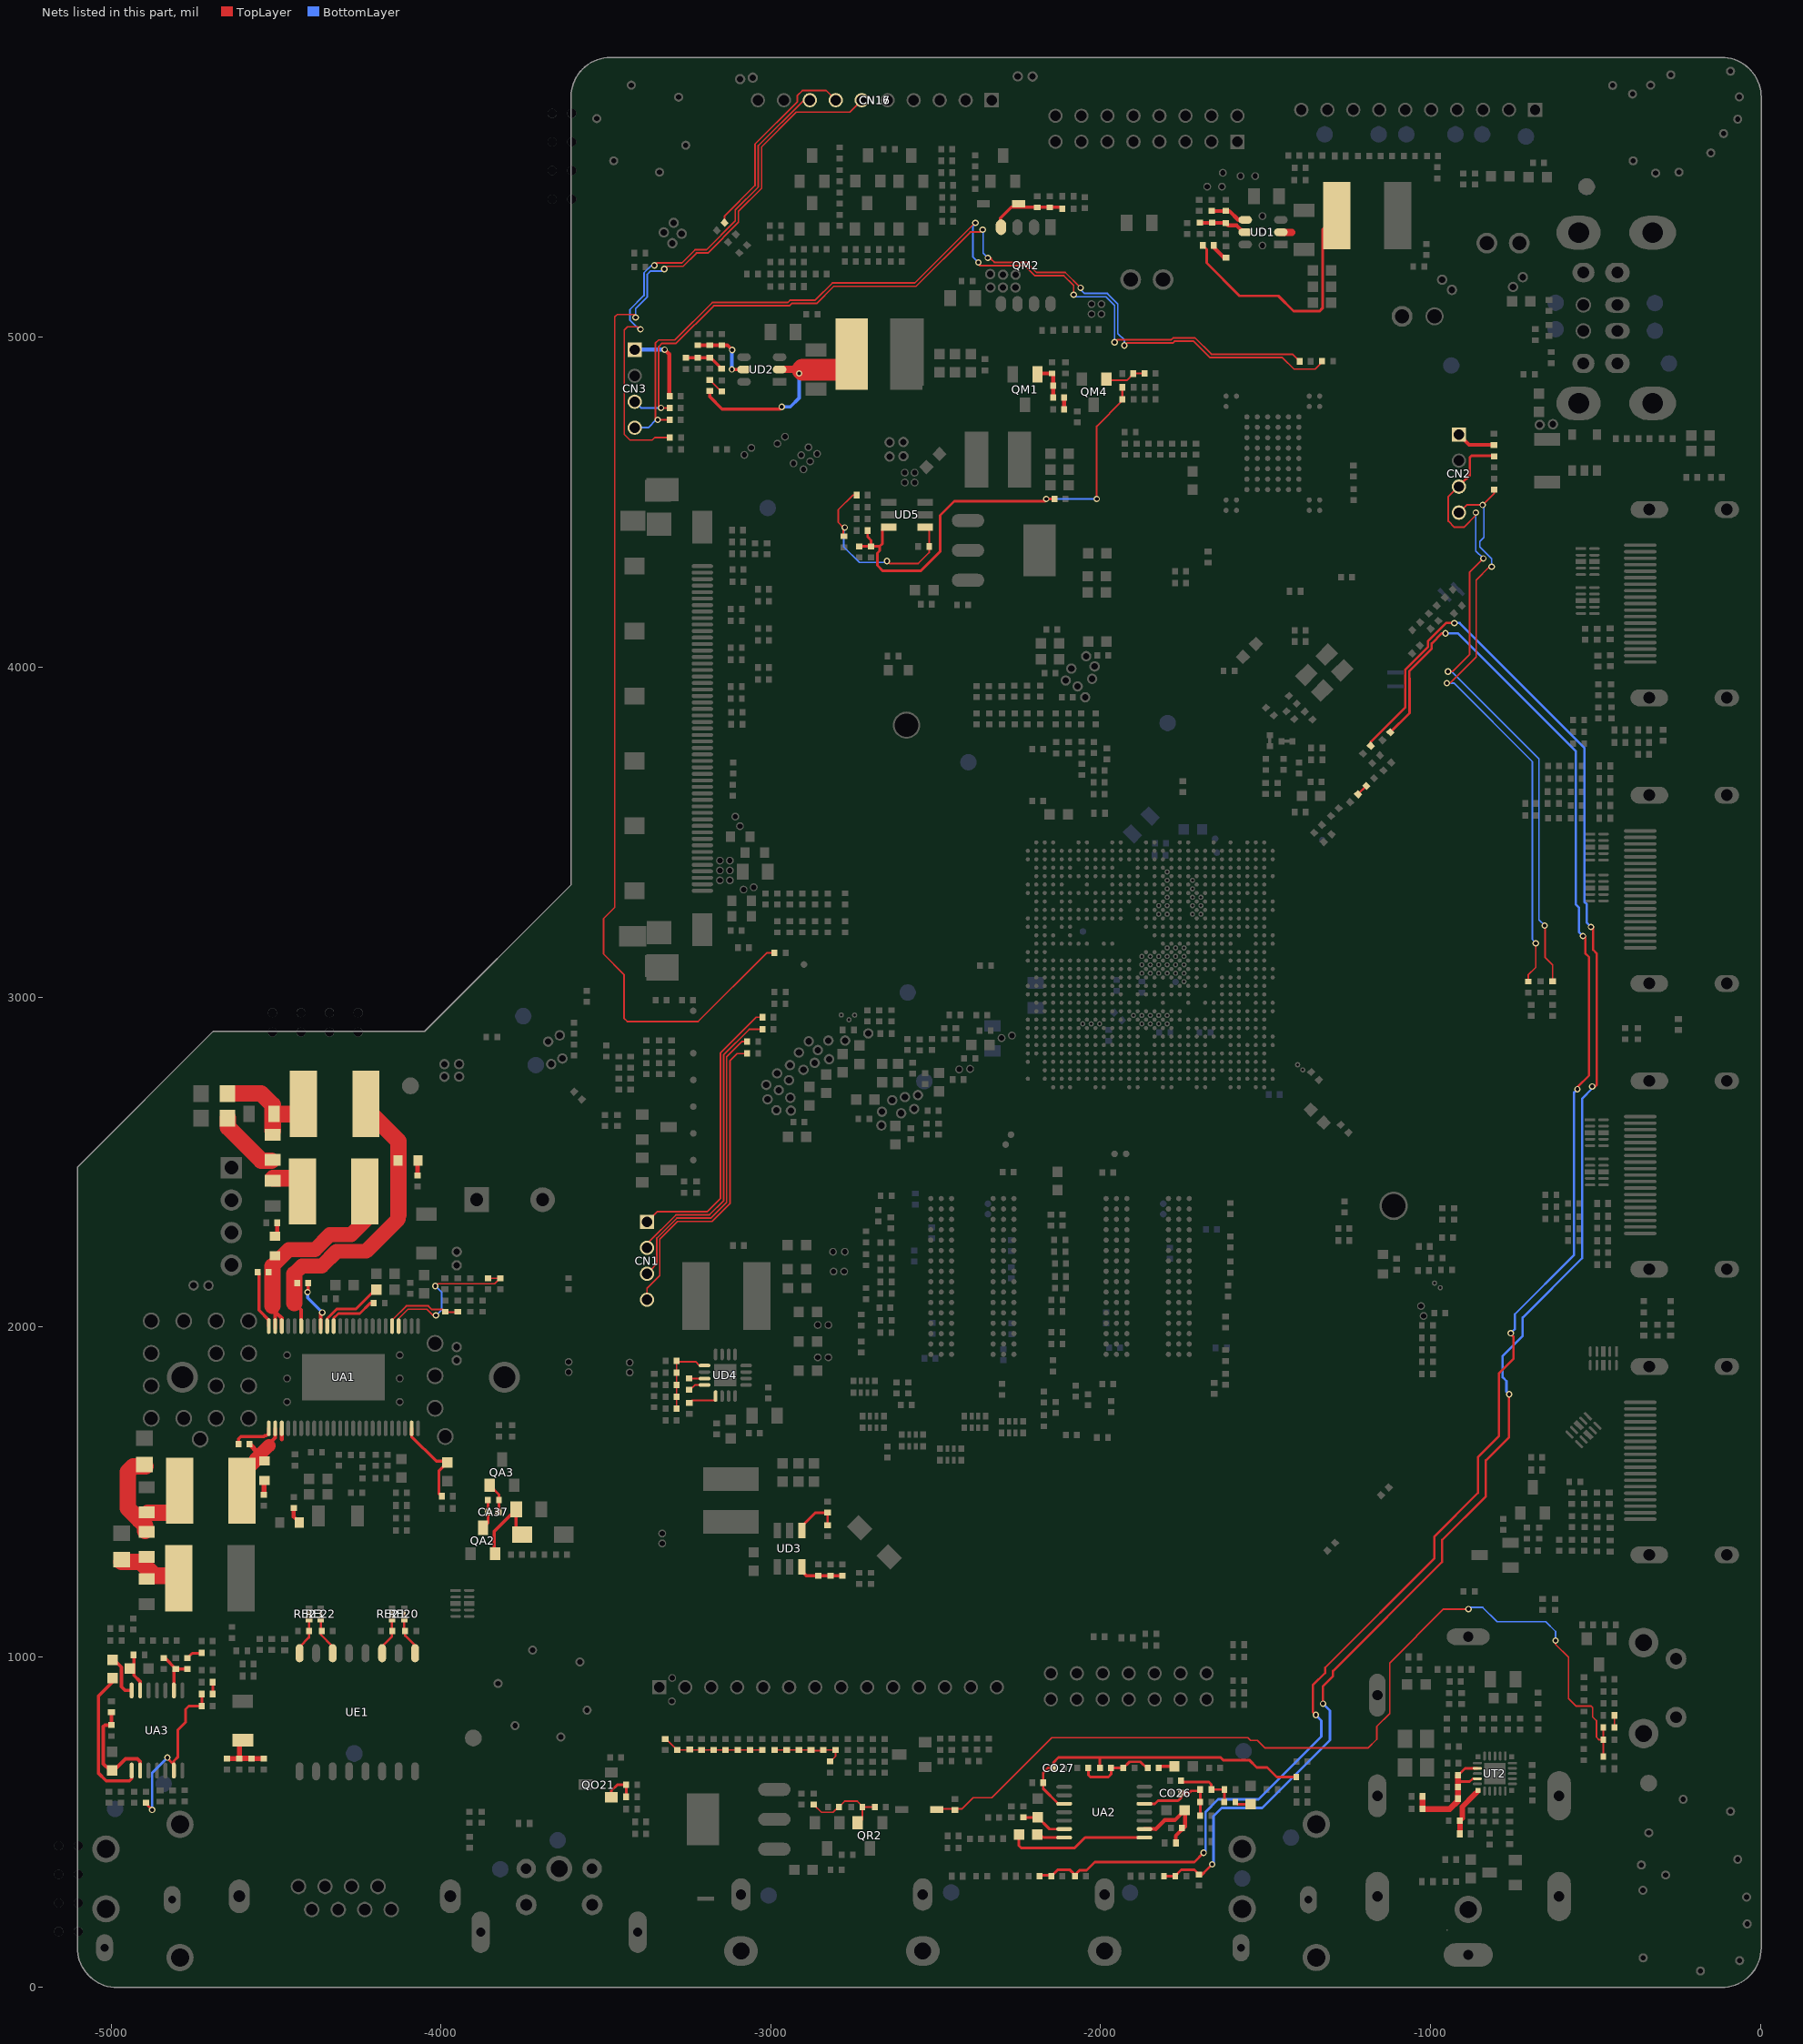
[diagram p0: the nets of this part, all layers, seen from the top]
# Altium PCB MISC86290.PcbDoc (part 25 of 31)
Units mil, origin at the board's own origin, x right, y up, seen from the top; angles counter-clockwise.
Board outline 5104.71 x 5851.49 mil, 2 copper layers (TopLayer, BottomLayer), stack 61.855 mil thick; 1026 components, 667 nets, 4280 pads, 2294 vias.

## Via types
v1: diameter 19.68, hole 11.81, TopLayer to BottomLayer, tented both sides, 1189 vias
v2: diameter 19.68/19.68 (per signal layer), hole 11.81, TopLayer to BottomLayer, tented both sides, 366 vias
v3: diameter 15.75, hole 7.87, TopLayer to BottomLayer, tented both sides, 348 vias
v4: diameter 23.62, hole 15.75, TopLayer to BottomLayer, tented both sides, 309 vias
v5: diameter 15.75/15.75 (per signal layer), hole 7.87, TopLayer to BottomLayer, tented both sides, 59 vias
v6: diameter 24/24 (per signal layer), hole 16, TopLayer to BottomLayer, tented both sides, 23 vias

## Nets (pads, with @x,y where several pads share a name; then routed paths per layer and width w, separated by ;. In a path a pad name is that pad's centre, name@x,y a point inside that pad or via, vN(x,y) a via of type N, cw(c..) or ccw(c..) an arc to the next point about the centre after c; other vN are vias at no path point) (continued)
NetCA14_1: CA14.1 CA18.2 LA1.2 RA30.1 | length 190.3
  TopLayer w50: RA30.1@-4968,1288.23 -4910.23,1288.23 -4868,1246 LA1.2@-4795.23,1246
NetCA17_1: CA17.1 CA18.1 LA2.2 RA31.1 | length 503.8
  TopLayer w50: CA18.1@-4897,1382.03 -4897,1398 -4912,1413 ; RA31.1@-4896,1577 -4899.01,1577 -4933,1577 -4949.17,1560.83 -4949.17,1450.17 -4914.5,1415.5 -4912,1413 ; LA2.2@-4791.88,1565.21 LA2.2@-4791.88,1503.52 -4791.88,1462.12 -4817,1437 -4888,1437 -4889.53,1435.47 -4912,1413
NetCA19_1: CA19.1 UA1.1 | length 129.8
  TopLayer w10: CA19.1@-4613.73,1645 -4613.73,1661.27 -4607,1668 -4536.43,1668 -4534.27,1670.17 -4529.51,1670.17 -4522.13,1677.55 UA1.1@-4522.13,1692.73
NetCA19_2: CA19.2 LA2.1 RA17.1 UA1.2 UA1.3 | length 203.6
  TopLayer w11.8: -4517.18,1649.37 -4502.44,1664.1 UA1.2@-4502.44,1692.73 ; -4482.76,1659.31 UA1.3@-4482.76,1692.73
  TopLayer w15: CA19.2@-4580.27,1645 -4554.69,1619.42
  TopLayer w40: LA2.1@-4577.55,1578.68 -4562.91,1593.33 -4562.91,1599.1 -4521.84,1640.17
NetCA20_1: CA20.1 CA21.2 UA1.23 | length 291.3
  TopLayer w9: UA1.23@-4089.06,1681.87 -4089.06,1668.06 -4014,1593 -3987.62,1593 CA21.2@-3981,1599.62 ; CA20.1@-3997.73,1487 -4006.5,1495.77 -4006.5,1563.12 CA21.2@-3981,1588.62
  TopLayer w10: UA1.23@-4089.06,1672.96 -4089.06,1681.87 UA1.23@-4089.06,1692.73
NetCA22_1: CA22.1 UA1.48 | length 171.5
  TopLayer w10: CA22.1@-4551.73,2162 -4551.73,2050.73 -4522.13,2021.13 UA1.48@-4522.13,2002.77
NetCA22_2: CA22.2 LA3.2 RA18.1 UA1.46 UA1.47 | length 714.5
  TopLayer w11.8: -4511,2064 -4511,2055.19 -4498.2,2042.39 ; UA1.47@-4502.44,1994.89 UA1.47@-4502.44,2023.63 ; UA1.47@-4502.44,2002.77 -4502.44,2038.15 -4498.2,2042.39 ; UA1.46@-4482.76,1994.89 UA1.46@-4482.76,2002.77 -4482.76,2026.94 -4498.2,2042.39
  TopLayer w45: -4511,2184.5 -4461,2234.5 -4382.23,2234.5 -4336.98,2279.75 -4272.25,2279.75 -4228.51,2323.49 LA3.2@-4228.51,2426.5
  TopLayer w50: -4511,2064 -4511,2184.5
NetCA23_1: CA23.1 UA1.38 | length 168.3
  TopLayer w8: UA1.38@-4325.28,2002.77 -4325.28,2026.84 -4311.12,2041 -4246,2041 -4215,2072 CA23.1@-4203.73,2072
  TopLayer w10: UA1.38@-4325.28,1994.89 UA1.38@-4325.28,1998.83
NetCA24_1: CA24.1 CA26.1 LA3.1 RA32.1 | length 291.5
  TopLayer w50: RA32.1@-4646,2633 -4646,2632.59 -4646,2605.5 -4544.5,2504 CA24.1@-4513.33,2504 ; CA26.1@-4508.77,2451.04 LA3.1@-4419.5,2451.04
NetCA24_2: CA24.2 CA27.1 LA4.2 RA33.1 | length 347.2
  TopLayer w50: -4618.5,2708 -4545,2708 -4510.36,2673.36 -4510.36,2646.5 CA24.2@-4510.36,2595 ; CA27.1@-4506.97,2645.5 -4505.97,2645.5 -4435,2645.5 -4413.49,2667.01 -4413.49,2676.38 LA4.2@-4413.49,2711
NetCA25_1: CA25.1 UA1.39 | length 209.9
  TopLayer w8: UA1.39@-4344.96,2002.77 -4344.96,2025.54 -4316.5,2054 -4258.57,2054 -4195.81,2116.76 CA25.1@-4195.81,2117
NetCA28_1: CA28.1 UA1.40 | length 160.4
  TopLayer w10: v1(-4404.27,2105.73) -4402.27,2105.73 CA28.1@-4402.27,2133 ; UA1.40@-4364.65,1994.89 UA1.40@-4364.65,2002.77 -4364.65,2039.35 v1(-4360,2044)
  BottomLayer w10: v1(-4404.27,2105.73) -4404.27,2088.27 v1(-4360,2044)
NetCA28_2: CA28.2 LA4.1 RA19.1 UA1.43 | length 917.2
  TopLayer w11: -4445,2072.84 -4423.7,2051.55 UA1.43@-4423.7,2002.77
  TopLayer w45: -4445,2161 -4421.5,2184.5 -4361.51,2184.5 -4316.27,2229.75 -4227.02,2229.75 -4129,2327.77 -4129,2339.95
  TopLayer w50: -4445,2072.84 -4445,2161 ; LA4.1@-4224.51,2645.95 -4211.95,2645.95 -4129,2563 -4129,2339.95
NetCA32_1: CA32.1 RA16.2 | length 50.2
  TopLayer w12: CA32.1@-4446.39,1450.79 -4446.39,1424.3 RA16.2@-4429.61,1407.52
NetCA33_1: CA33.1 RA17.2 | length 37.5
  TopLayer w15: CA33.1@-4536.39,1499.52 RA17.2@-4536.39,1537.01
NetCA34_1: CA34.1 RA18.2 | length 33.5
  TopLayer w12: RA18.2@-4496.04,2282.52 CA34.1@-4496.04,2316.01
NetCA35_1: CA35.1 RA19.2 | length 44.5
  TopLayer w15: CA35.1@-4071,2459.73 RA19.2@-4071,2504.22
NetCA36_2: CA36.2 DA9.K QA2.E | length 248.8
  TopLayer w10: QA2.E@-3838.5,1308 -3838.5,1380.53 CA36.2@-3772.03,1447 -3772.03,1386.04 DA9.K@-3756.99,1371
NetCA37_1: CA37.1 QA2.C RA23.1 | length 90.1
  TopLayer w8: QA2.C@-3872.5,1391.03 -3857.73,1405.8 CA37.1@-3857.73,1439 RA23.1@-3857.73,1475
NetCA37_2: CA37.2@-3824.26,1439 CA37.2@-3831.15,1439 QA3.B RA23.2 | length 92.7
  TopLayer w8: QA3.B@-3852.5,1520 -3824.27,1491.77 RA23.2@-3824.27,1475 CA37.2@-3824.26,1439
NetCA38_2: CA38.2 RA14.2 UA1.29 | length 243
  TopLayer w5: UA1.29@-4148.11,2002.77 -4148.11,2021.89 -4145,2025 -4144.18,2025 -4105.18,2064 -4038.14,2064 -4027.14,2053 -3993.73,2053 CA38.2@-3987,2046.27 ; CA38.2@-3987,2045.27 RA14.2@-3949,2045.27
NetCA39_2: CA39.2 RA12.2 UA1.28 | length 508.6
  TopLayer w5: UA1.28@-4128.43,2002.77 -4128.43,2025.57 -4100,2054 -4043,2054 -4024,2035 v1(-4015,2035) v1@-4015,2040 ; v1(-4017,2124) -4010,2131 -3837.11,2131 CA39.2@-3820.35,2147.76 RA12.2@-3857.35,2147.76
  BottomLayer w5: v1(-4017,2124) -3997.66,2104.66 -3997.66,2052.34 v1(-4015,2035)
NetCA53_2: CA53.2 RO31.2 RO33.1 UA3.2 | length 153.7
  TopLayer w10: RO33.1@-4840.84,996.73 -4837.3,996.73 CA53.2@-4803.84,963.27 ; UA3.2@-4809.73,898.32 -4809.73,957.37 CA53.2@-4803.84,963.27 ; RO31.2@-4768.34,963.27 CA53.2@-4803.84,963.27
NetCA56_2: CA56.2 RO32.2 RO34.1 UA3.13 | length 531.3
  TopLayer w8: RO34.1@-4892.77,559 RO34.1@-4894.5,557.27 -4894.5,555 v1(-4875.5,536) ; v1(-4829.5,694.5) -4829.5,692.68 UA3.13@-4809.73,672.92 ; UA3.13@-4809.73,655.21 UA3.13@-4809.73,672.92 ; CA56.2@-4725.25,851 -4765,851 -4774.5,841.5 -4774.5,801.75 -4797.14,779.1 -4797.14,696.86 -4809.73,684.27 UA3.13@-4809.73,672.92 ; CA56.2@-4724.98,851 RO32.2@-4724.98,887.15
  BottomLayer w8: v1@-4877,537.5 v1(-4875.5,536) -4875.5,648.5 v1(-4829.5,694.5)
NetCD4_1: CD4.1 RD1.2 RD2.2 UD1.5 | length 149.3
  TopLayer w12: RD1.2@-1699.47,5347.46 -1621.75,5347.46 CD4.1@-1621.02,5346.73 -1613.61,5339.32 -1587.57,5339.32 -1567.17,5318.92 UD1.5@-1562.04,5318.92
NetCD5_1: CD5.1 RD3.2 | length 50
  TopLayer w12: CD5.1@-1657.52,5273 -1626.78,5242.27 RD3.2@-1620.25,5242.27
NetCD5_2: CD5.2 LD1.1 LD4.1 UD1.2 | length 832.5
  TopLayer w8: CD5.2@-1690.73,5279 -1679,5267.27 -1679,5226 -1579,5126 -1461.25,5126 -1415.25,5080 -1336.05,5080 -1327.5,5088.55 -1327.5,5326.27 LD4.1@-1284.77,5369 ; LD4.1@-1269.77,5348 LD4.1@-1252.25,5330.48
  TopLayer w21.6: UD1.2@-1457,5317.92 -1420.79,5317.92
NetCD6_2: CD6.2 RD4.1 UD1.4 | length 112.8
  TopLayer w12: RD4.1@-1663.25,5384.27 -1662.25,5383.27 CD6.2@-1621.25,5383.27 -1610.04,5383.27 -1583.09,5356.32 UD1.4@-1562.04,5356.32
NetCD14_1: CD14.1 LD2.2 LD3.1 UD2.2 | length 614.1
  TopLayer w10: CD14.1@-3185.25,4837.27 -3185.25,4820.4 -3147.85,4783 -2971.5,4783 -2967,4787.5 v1(-2967,4789.5)
  TopLayer w21.6: UD2.2@-2973.28,4902.85 -2910.3,4902.85
  TopLayer w65: -2904.3,4901.88 LD3.1@-2746.25,4901.88
  BottomLayer w10: v1(-2967,4789.5) -2941,4789.5 -2914.25,4816.25 v1(-2914.25,4891)
NetCD14_2: CD14.2 RD13.2 | length 51.3
  TopLayer w5: CD14.2@-3185.25,4870.73 -3150.78,4836.27 RD13.2@-3148.25,4836.27
NetCD15_1: CD15.1 RD14.2 RD15.2 RD16.2 | length 122.1
  TopLayer w10: CD15.1@-3257.25,4938 -3221.71,4938 RD15.2@-3221.25,4938.46 RD16.2@-3185.25,4938.46 -3182.71,4938.46 RD14.2@-3149.25,4905
NetCD22_1: CD22.1 RD21.1 UD3.1 | length 153.4
  TopLayer w8: UD3.1@-2905.85,1368.12 UD3.1@-2905.85,1375.15 ; UD3.1@-2905.85,1383.12 -2905.85,1395.96 -2864.54,1437.27 CD22.1@-2828,1437.27 RD21.1@-2828,1398.73
NetCD23_1: CD23.1 RD22.1 RD23.2 UD3.6 | length 141.5
  TopLayer w10: UD3.6@-2905.85,1272.88 -2905.85,1259.6 -2892.52,1246.27 RD23.2@-2856.25,1246.27 -2783.52,1246.27 CD23.1@-2783.25,1246.53
NetCD29_1: CD29.1 RD11.2 RD12.2 UD2.5 | length 206.9
  TopLayer w10: RD11.2@-3222,4976.27 -3131.52,4976.27 v1(-3117.25,4962) ; v1(-3118.25,4902.85) UD2.5@-3081.55,4902.85
  BottomLayer w10: v1(-3118.25,4902.85) -3118.25,4961 v1(-3117.25,4962)
NetCD34_2: CD34.2 UD4.9 | length 98.3
  TopLayer w5: CD34.2@-3247.25,1769.73 -3239.89,1777.09 UD4.9@-3167.54,1777.09 ; UD4.9@-3169.43,1777.09 UD4.9@-3167.54,1777.09 ; UD4.9@-3167.54,1790.7 UD4.9@-3167.54,1777.09
NetCD35_1: CD35.1 UD4.8 | length 53
  TopLayer w5: CD35.1@-3248.25,1810.27 -3244.73,1810.27 -3230.84,1824.16 UD4.8@-3201,1824.16
NetCD35_2: CD35.2 UD4.7 | length 56.8
  TopLayer w5: CD35.2@-3248.25,1843.73 -3248.13,1843.85 UD4.7@-3201,1843.85 UD4.7@-3210.51,1843.85
NetCD36_1: CD36.1 RD32.1 RD34.1 RD36.1 RD38.1 UD4.5 | length 231.1
  TopLayer w5: RD32.1@-3285.77,1753.5 RD36.1@-3285.77,1788.5 CD36.1@-3285.77,1897 ; CD36.1@-3283.77,1895 -3228.25,1895 -3216.46,1883.22 UD4.5@-3201,1883.22
NetCD52_1: CD52.1 RD51.1 RD52.1 UD5.1 | length 608.9
  TopLayer w5: RD51.1@-2780.5,4396.73 RD51.1@-2780.5,4398.97 ; v1@-2779.25,4423 -2795.5,4439.25 -2795.5,4477.5 -2751,4522 RD52.1@-2739.98,4522 ; RD51.1@-2776.86,4395.33 RD51.1@-2780.5,4398.97 ; v1(-2775.84,4423.76) -2780.5,4419.1 RD51.1@-2780.5,4398.97 ; v1(-2648,4322) -2640.5,4314.5 -2553.17,4314.5 -2520,4347.67 -2520,4362.5 CD52.1@-2524.23,4366.73 ; UD5.1@-2531.88,4425.1 -2519.77,4412.98 CD52.1@-2519.77,4366.23
  BottomLayer w5: v1@-2779.25,4423 -2779.25,4365.44 -2731.81,4318 -2652,4318 v1(-2648,4322)
NetCD53_1: CD53.1 RD53.1 RD54.2 RD57.2 RD60.2 RF56.2 UD5.6 | length 1469.1
  TopLayer w5: v1(-2012,4510.43) -2012,4730.64 -1933.98,4808.66 RD57.2@-1933.98,4811.95
  TopLayer w7: RD57.2@-1933.98,4811.95 RF56.2@-1933.98,4848.95
  TopLayer w8: RD60.2@-2732.5,4366.5 RD53.1@-2696,4366.5 ; RD54.2@-2706.7,4414.58 -2706.7,4395.7 -2696,4385 RD53.1@-2696,4366.5 ; UD5.6@-2644,4423.22 UD5.6@-2642.12,4425.1 -2654.86,4425.1 -2662,4417.96 -2662,4374.29 -2669.79,4366.5 ; v1@-2168.72,4503.78 -2443.68,4503.78 -2486.4,4461.06 -2486.4,4350.87 -2544.27,4293 -2661.5,4293 -2677.16,4308.66 -2677.16,4346 -2669.79,4353.37 -2669.79,4366.5 ; v1@-2162.57,4509.93 CD53.1@-2140.43,4509.93 ; RD53.1@-2696,4366.5 -2669.79,4366.5
  BottomLayer w5: v1(-2165.07,4510.43) v1(-2012,4510.43)
NetCE1_2: CE1.2 RE20.2 RE20.3 UE1.1 | length 114.6
  TopLayer w7: CE1.2@-4111.5,1078.77 RE20.2@-4111.5,1113.29 ; CE1.2@-4108.5,1078.77 -4108.5,1064.47 -4078.5,1034.47 UE1.1@-4078.5,1011.13
NetCE2_2: CE2.2 RE21.2 RE21.3 UE1.3 | length 114.5
  TopLayer w7: UE1.3@-4178.5,1011.13 -4178.5,1032 -4148.53,1061.97 RE21.2@-4148.53,1113.26
NetCE3_2: CE3.2 RE22.2 RE22.3 UE1.6 | length 117.1
  TopLayer w7: RE22.2@-4364.5,1113.29 -4364.5,1068 -4328.5,1032 UE1.6@-4328.5,1011.13
NetCE4_2: CE4.2 RE23.2 RE23.3 UE1.8 | length 114
  TopLayer w7: UE1.8@-4428.5,1011.13 -4428.5,1030 -4400,1058.5 RE23.2@-4400,1113.29
NetCE5_1: CE5.1 RE1.1 RE2.1 RE3.1 RE4.1 | length 210.4
  TopLayer w15: RE4.1@-4648.5,691.96 -4648.31,691.78 RE3.1@-4610.83,691.78 ; RE3.1@-4610.83,694.07 RE3.1@-4610.83,693.18 ; CE5.1@-4600.95,747.44 -4611.33,737.07 -4611.33,693.18 RE3.1@-4610.83,693.18 ; RE1.1@-4574.17,691.96 -4575.38,693.18 RE3.1@-4610.83,693.18 ; RE2.1@-4536.67,691.78 RE3.1@-4610.83,691.78 ; RE3.1@-4610.83,691.78 RE3.1@-4610.83,693.18
NetCI2_1: CI2.1 RI1.2 | length 35.8
  TopLayer w7: CI2.1@-1220.17,3614.83 RI1.2@-1194.83,3640.17
NetCI3_2: CI3.2 CI4.1 RI3.2 RI4.2 | length 5399.8
  TopLayer w7: v1(-1348,824) -1357,833 -1357,913.82 -1319.49,951.33 -1319.49,967.32 -989.09,1297.72 -989.09,1364.02 -856.28,1496.83 -856.28,1605.51 -792.34,1669.45 -792.34,1859.6 -749,1902.94 -749,1971 -757,1979 v1(-757,1981) ; -1064,3967 -1064,3988.55 -996.34,4056.21 -996.34,4072.15 -965.5,4103 v1(-955,4103) ; v1(-555,2721) -555,2727.14 -519.66,2762.48 -519.66,3121.72 -531.34,3133.4 -531.34,3183.34 -533,3185 v1(-538,3185)
  TopLayer w8: RI3.2@-2185.27,338 -2146.55,338 -2130.71,353.84 -2092.84,353.84 -2078,339 -2064,353 -2043,353 -2018,378 -1716,378 v1(-1688,406) ; CI4.1@-1122.17,3802.83 -1064,3861 -1064,3967
  BottomLayer w7: v1(-955,4103) -917.03,4103 -560,3745.97 -560,3281.16 -550.34,3271.5 -550.34,3197.34 v1(-538,3185) ; v1(-757,1981) -744.54,1993.46 -744.54,2038.63 -565,2218.18 -565,2711 v1(-555,2721)
  BottomLayer w8: v1(-1688,406) -1682,412 -1682,529.85 -1643.85,568 -1521.15,568 -1331,758.15 -1331,807 v1(-1348,824)
NetCI5_2: CI5.2 CI6.1 RI5.2 RI6.2 | length 5224.2
  TopLayer w7: v1(-1326,858) -1326,910.87 -1295.49,941.39 -1295.49,957.38 -965.09,1287.77 -965.09,1354.08 -832.28,1486.89 -832.28,1595.57 -762,1665.85 v1(-762,1796) ; CI6.1@-1181.17,3761.83 -1181.17,3774.33 -1076.5,3879 -1076.5,3993.02 -1008.34,4061.18 -1008.34,4078.72 -953.06,4134 v1(-928,4134) ; v1(-514,3213) -507.34,3213 -507.34,3143.34 -495.66,3131.66 -495.66,2734.6 -501.15,2729.11 v1(-510.12,2729.11)
  TopLayer w8: RI6.2@-1808.27,335 -1774.73,335 -1755.73,354 -1716.27,354 CI5.2@-1702,339.73 -1693.27,339.73 -1678.69,354.31 ; -1687.27,345.73 -1678.69,354.31 ; v2(-1662,371) -1678.69,354.31
  BottomLayer w7: v1(-928,4134) -912.03,4134 -534,3755.97 -534,3289.1 -526.34,3281.44 -526.34,3225.34 v1(-514,3213) ; v1(-762,1796) -770,1804 -770,1836.06 -781.34,1847.4 -781.34,1912.22 -720.54,1973.02 -720.54,2028.69 -541,2208.24 -541,2692 -510.12,2722.88 v1(-510.12,2729.11)
  BottomLayer w8: v2@-1658,371 -1658,517.08 -1633.08,542 -1510.38,542 -1305,747.38 -1305,837 v1(-1326,858)
NetCK3_2: CK3.2 DK10.K RK29.1 RK30.2 RK31.1 RK32.1 RK33.2 RK34.1 RK36.1 | length 308
  TopLayer w5: RK34.1@-3320.25,751 -3317.52,751 RK33.2@-3284.06,717.53 RK36.1@-3137.25,717.53 RK31.1@-3100.19,717.53 RK30.2@-3063.13,717.53 RK29.1@-3026.07,717.53
NetCK9_2: CK9.2 DK9.K RK24.1 RK26.2 RK27.1 RK28.1 RK35.1 | length 228.4
  TopLayer w5: RK28.1@-2989,717.53 RK27.1@-2951.94,717.53 RK35.1@-2914.88,717.53 -2878.47,717.53 -2876.74,715.81 -2842.48,715.81 CK9.2@-2840.75,717.53 RK26.2@-2803.64,717.53 -2803.64,699.09 RK24.1@-2820,682.73
NetCM1_2: CM1.2 QM4.B RM1.2 | length 119.6
  TopLayer w5: QM4.B@-1982.75,4874 -1978.75,4870 -1920.78,4870 RM1.2@-1900.78,4890 ; RM1.2@-1903.33,4891 -1875.65,4891
NetCM2_1: CM2.1 RM4.2 | length 36
  TopLayer w12: CM2.1@-2110.77,4781.5 RM4.2@-2110.77,4817.5
NetCM4_1: CM4.1 QM1.G RM3.2 RM4.1 | length 120.1
  TopLayer w12: QM1.G@-2191.6,4888.24 -2189.04,4890.81 CM4.1@-2147,4890.81 -2144.23,4888.04 RM3.2@-2144.23,4854 RM4.1@-2144.23,4817.5
NetCM15_1: CM15.1 CM16.1 DM11.K QM2.4 RM14.2 | length 230.7
  TopLayer w10: QM2.4@-2304.25,5324.14 -2304.25,5361.85 -2271.1,5395 -2124.98,5395
NetCN1_1: CN1.1 R202.1 | length 865
  TopLayer w5: CN1.1@-3375.25,2318.74 -3343.99,2350 -3192,2350 -3152.91,2389.09 -3152.91,2830.12 -3044.02,2939 R202.1@-3025.5,2939
NetCN1_2: CN1.2 R203.1 | length 889.7
  TopLayer w5: CN1.2@-3375.25,2240 -3375.25,2252.43 -3287.67,2340 -3186,2340 -3143.91,2382.09 ; -3143.41,2382.59 -3143.41,2824.59 -3065.5,2902.5 R203.1@-3025.5,2902.5
NetCN1_3: CN1.3 R204.1 | length 894.6
  TopLayer w5: CN1.3@-3375.25,2172.26 -3364.69,2172.26 -3345.75,2191.2 -3345.75,2269.34 -3285.09,2330 -3181.86,2330 -3133.91,2377.95 -3133.91,2818.59 -3086.98,2865.52 R204.1@-3071.72,2865.52
NetCN1_4: CN1.4 R205.1 | length 951.3
  TopLayer w5: CN1.4@-3375.25,2082.52 -3375.25,2117.25 -3336.75,2155.75 -3336.75,2265.75 -3282.5,2320 -3177.72,2320 -3123.91,2373.81 -3123.91,2807.09 -3101.98,2829.02 R205.1@-3071.72,2829.02
NetCN2_1: CN2.1 R137.1 | length 118.8
  TopLayer w12: CN2.1@-914,4705.11 -883.16,4674.27 R137.1@-808,4674.27
NetCN2_3: CN2.3 R139.1 R140.1 | length 2033.5
  TopLayer w5: v1(-947,3987) -933.79,3987 -881.5,4039.29 -881.5,4288.5 v1(-840,4330) ; CN2.3@-914,4549.63 CN2.3@-915,4548.63 ; CN2.3@-905.05,4558.58 CN2.3@-915,4548.63 ; v1(-862.82,4468.89) -862.82,4460.77 -898.88,4424.7 -927.95,4424.7 -946.25,4443 -946.25,4517.38 CN2.3@-915,4548.63 ; v1(-654,3217) v1@-653,3218 ; v1@-653,3217 -653,3120.71 -630,3097.71 R140.1@-630,3047.73
  TopLayer w8: CN2.3@-905.05,4558.58 -881.03,4582.6 -881.03,4636.09 -875.89,4641.23 -808.5,4641.23 R139.1@-807,4639.73
  BottomLayer w5: v1(-947,3987) -936.56,3987 -671.34,3721.79 -671.34,3234.34 v1(-654,3217) ; v1(-862.82,4468.89) -862.82,4352.82 v1(-840,4330)
NetCN2_4: CN2.4 R138.1 R141.1 | length 1808
  TopLayer w5: v1(-950.89,3952) -940.51,3952 -861.5,4031.01 -861.5,4264.5 -821,4305 v1(-815,4305) ; CN2.4@-914,4468.89 -890.89,4492 v1(-842,4492) -807,4527 R138.1@-807,4538.27 ; R141.1@-704,3047.23 -704,3067 -681,3090 v1(-681,3163)
  BottomLayer w5: v1(-950.89,3952) -929.84,3952 -691.34,3713.5 -691.34,3175.34 -681,3165 v1(-681,3163) ; v1(-842,4492) -838.34,4488.34 -838.34,4393.32 -850.59,4381.07 -850.59,4365.12 -815,4329.53 v1(-815,4305)
NetCN3_1: CN3.1 R171.1 | length 234.1
  TopLayer w12: v1(-3321.95,4963) -3308,4949.05 R171.1@-3308,4829.14 ; R171.1@-3308,4822.37 -3308,4824.14 R171.1@-3306.23,4822.37
  BottomLayer w12: CN3.1@-3412.11,4963 v1(-3321.95,4963)
NetCN3_3: CN3.3 R31.1 R72.1 | length 2725.9
  TopLayer w5: v1@-3340,4786.5 -3340,4972.1 -3330,4982.1 -3287.12,4982.1 -3173.23,5096 -2943.57,5096 -2936.57,5103 -2861.33,5103 -2809.33,5155 -2559.78,5155 -2395.28,5319.5 -2364.94,5319.5 ; v1(-3333,4786.5) -3332.87,4786.37 R31.1@-3306.23,4786.37 ; -2331.5,5241 -2331.5,5236.5 -2322.5,5227.5 -2225.5,5227.5 -2195,5197 -2107.5,5197 v1(-2061,5150.5) ; -1920.34,4983.16 -1781.57,4983.16 -1776.24,4988.49 -1718.14,4988.49 -1668.65,4939 -1449,4939 -1414,4904 -1349.5,4904 -1328.73,4924.77 R72.1@-1328.73,4928
  BottomLayer w5: CN3.3@-3412.5,4805.13 -3393.87,4786.5 v1(-3333,4786.5) ; v1@-2356.5,5325.74 -2356.5,5255.26 v1(-2342.39,5241.16) ; v1@-2061,5145.5 -2048.66,5133.16 -1979.47,5133.16 -1948,5101.69 -1948,5012 -1928,4992 v1(-1928,4975.5)
  other v1: -2357.6,5326.84
NetCN3_4: CN3.4 R30.1 R73.1 | length 2758.6
  TopLayer w5: v1@-3350,4750.5 -3350,4982.3 -3340.19,4992.1 -3291.26,4992.1 -3177.37,5106 -2947.72,5106 -2940.72,5113 -2865.48,5113 -2813.48,5165 -2563.92,5165 v1@-2381.87,5347.05 ; v1(-3343,4750.5) -3342.87,4750.37 R30.1@-3306.23,4750.37 ; -2367,5217.5 -2229.64,5217.5 -2199.14,5187 -2111.64,5187 -2082.18,5157.54 v1(-2082.18,5129.34) ; -1950.34,4993.16 -1785.71,4993.16 -1780.38,4998.49 -1714,4998.49 -1664.51,4949 -1418.23,4949 R73.1@-1396.73,4927.5
  BottomLayer w5: CN3.4@-3412.5,4726.39 -3371.48,4726.39 -3347.37,4750.5 v1(-3343,4750.5) ; v1@-2379.66,5345.34 -2387,5338 -2387,5243.5 v1(-2371,5227.5) ; v1@-2076,5123.16 -1983.61,5123.16 -1958,5097.55 v1(-1958,4985.5)
  other v1: -2379.66,5347.05
NetCN16_6: CN16.6 CN17.6 RG43.1 | length 3895.8
  TopLayer w5: v1(-3410,5060.5) -3410,5067 -3412.5,5069.5 -3465.61,5069.5 -3473.11,5062 -3473.11,3272.17 -3507.13,3238.15 -3507.13,3130.57 -3445.34,3068.77 -3445.34,2936.2 -3435.14,2926 -3220.36,2926 -3011.86,3134.5 RG43.1@-2988.73,3134.5 ; v1(-3323,5207.5) -3314.66,5215.84 -3265.72,5215.84 -3225.56,5256 -3191,5256 -3098.09,5348.91 -3098.09,5381.9 -3028,5451.99 -3028,5577.5 -2922.65,5682.85 -2760.98,5682.85 CN16.6@-2724.37,5719.46
  BottomLayer w5: v1(-3410,5060.5) -3410,5087.14 -3374.5,5122.64 -3374.5,5191.5 -3365.26,5200.74 -3327.76,5200.74 -3322,5206.5 v1(-3323,5207.5)
NetCN16_7: CN16.7 CN17.7 RG41.1 | length 611.8
  TopLayer w5: RG41.1@-3140.17,5347.83 -3140.17,5368.11 -3048,5460.28 -3048,5585.78 -2919.5,5714.28 -2919.5,5733.5 -2904.39,5748.61 -2832.26,5748.61 CN16.7@-2803.11,5719.46
NetCN16_8: CN16.8 CN17.8 RG44.1 | length 1508.1
  TopLayer w5: -3402.6,5032.1 -3434.78,5032.1 -3444.11,5022.77 -3444.11,4706.11 -3427,4689 -3359.5,4689 -3352,4696.5 RG44.1@-3306,4696.5 RG44.1@-3308.5,4699 ; -3345.66,5225.84 -3269.86,5225.84 -3229.71,5266 -3195.14,5266 -3108.09,5353.05 -3108.09,5386.05 -3038,5456.14 -3038,5581.64 -2900.19,5719.46 CN16.8@-2881.85,5719.46
  BottomLayer w5: v1@-3398.53,5024.5 -3427.34,5053.32 -3427.34,5083.94 -3384.5,5126.78 -3384.5,5195.64 v1@-3361.64,5218.5
  other v1: -3395,5024.5 -3353,5218.5
NetCO13_1: CO13.1 RO11.1 | length 49.5
  TopLayer w10: RO11.1@-1823.77,663.01 -1818.28,668.5 CO13.1@-1776.5,668.5
NetCO14_1: CO14.1 RO12.1 | length 40
  TopLayer w8: RO12.1@-1585.46,553.19 CO14.1@-1545.5,553.19
NetCO15_2: CO15.2 RO11.2 RO13.1 RO55.1 | length 241.8
  TopLayer w8: RO55.1@-2037.5,663 -2037.5,642 -2031.5,636 -1976.5,636 -1968.77,643.73 RO13.1@-1968.77,663.01 CO15.2@-1931.23,663 -1912.39,681.84 -1879.91,681.84 -1861.07,663.01 RO11.2@-1857.23,663.01
NetCO16_2: CO16.2 RO12.2 RO14.1 RO56.1 | length 189.6
  TopLayer w8: RO56.1@-1756.27,624.5 -1751.93,620.16 -1672,620.16 -1664.77,612.93 RO14.1@-1664.77,597.86 CO16.2@-1625,597.85 -1625.23,597.62 RO12.2@-1625.23,559.5
NetCO17_1: CO17.1 CO18.1 UA2.6 | length 141.5
  TopLayer w8: CO18.1@-2234,513.27 CO17.1@-2195.73,513.27 ; CO17.1@-2193,521 -2193,516 -2154.82,477.82 UA2.6@-2110.55,477.82
NetCO19_1: CO19.1 UA2.7 | length 88
  TopLayer w8: CO19.1@-2191.19,470 -2173.42,452.23 UA2.7@-2110.55,452.23
NetCO19_2: CO19.2 UA2.8 | length 441.3
  TopLayer w8: CO19.2@-2247.81,461 -2247.81,427.81 -2241,421 -2078.59,421 -2047.36,452.23 UA2.8@-1867.44,452.23 ; CO19.2@-2246.81,458 CO19.2@-2246.81,470
NetCO20_2: CO20.2 CO21.2 LO2.1 UA2.9 | length 256.8
  TopLayer w11: UA2.9@-1867.44,477.82 -1833.18,477.82
  TopLayer w12: -1833.18,477.82 -1806,505 -1775.19,505 CO20.2@-1745.19,535 -1744.41,534.22 -1744.41,485.33 -1772.27,457.47 LO2.1@-1772.27,436
NetCO25_2: CO25.2 QO21.B RO27.1 | length 109.1
  TopLayer w8: QO21.B@-3483.5,574.5 -3483.5,594.02 -3465.02,612.5 CO25.2@-3438.52,612.5 RO27.1@-3438.52,575.53
NetCO26_1: CO26.1 RO14.2 RO16.1 RO58.2 UA2.12 | length 270.4
  TopLayer w8: UA2.12@-1867.44,554.59 -1835.91,554.59 -1826.5,564 -1765,564 -1756.27,572.73 CO26.1@-1756.27,587 ; CO26.1@-1756.27,587 -1732.56,586.94 -1726,593.5 -1698.23,593.5 RO58.2@-1698.23,559.5 RO16.1@-1698.23,518 ; RO58.2@-1697.73,555.5 RO58.2@-1697.73,556.73
NetCO27_1: CO27.1 RO13.2 RO15.1 RO57.2 UA2.3 | length 980.8
  TopLayer w8: UA2.3@-2110.55,554.59 -2128.59,554.59 -2174.5,600.5 RO57.2@-2174.5,618.5 -2174.5,648.12 -2159.61,663 CO27.1@-2143.73,663 -2143.73,678.89 -2127.77,694.84 -1675.5,694.84 ; RO13.2@-2002.23,663.01 -2002.23,692.61 ; -1675.5,694.82 -1636.7,694.82 -1629.13,687.25 -1549.65,687.25 -1527.4,665 -1495.6,665 -1465.96,635.36 RO15.1@-1407.14,635.36
NetCO33_2: CO33.2 RO31.1 | length 40.8
  TopLayer w8: RO31.1@-4768.34,996.73 -4754.07,1011 CO33.2@-4733.43,1011
NetCO34_2: CO34.2 RO32.1 | length 36.2
  TopLayer w8: RO32.1@-4691.78,887.15 CO34.2@-4691.78,923.34
NetCO35_1: CO35.1 UA3.7 | length 130.8
  TopLayer w10: CO35.1@-4995,990.81 -4990.31,990.81 -4968.56,969.06 -4968.56,909.06 -4957.82,898.32 UA3.7@-4937.69,898.32
NetCO35_2: CO35.2 UA3.8 | length 443.4
  TopLayer w10: CO35.2@-4995,935.19 -4995,924.5 -5038.75,880.75 -5038.75,648.25 -5014.5,624 -4944.5,624 -4937.69,630.81 UA3.8@-4937.69,655.21
NetCO36_2: CO36.2 CO37.2 LO3.1 UA3.9 | length 342.1
  TopLayer w11: LO3.1@-4999,832.27 -4999,793.24 -5018.77,793.23 -5023.25,788.75 -5023.25,676.09 -5003.34,656.19 CO36.2@-4997,656.19 -4990.31,656.19 -4956,690.5 -4919.86,690.5 -4912.1,682.74 UA3.9@-4912.1,655.21
NetCO41_1: CO41.1 CO42.1 UA3.6 | length 115.4
  TopLayer w10: CO42.1@-4930.73,1006 -4930.73,944.05 -4912.1,925.42 UA3.6@-4912.1,898.32
NetCR1_1: CR1.1 CR4.2 DR3.K RR10.1 RR11.2 | length 2808.7
  TopLayer w5: DR3.K@-2496.85,539 -2421,539 -2387,573 -2330.67,573 -2148.67,755 -1553.75,755 -1545.5,746.75 -1525,746.75 -1501.75,723.5 -1189.55,723.5 -1163,750.05 -1163,789.25 -1123.92,828.33 -1123.92,981.33 -960.41,1144.84 v1(-885.11,1144.84) ; v1(-621,1049.5) -621,1038 -582,999 -582,873.5 -559.5,851 -513.5,851 -508.5,846 -508.5,817.77 -497,806.27 -497,756.5 -489,748.5 CR4.2@-476.23,748.5 ; RR10.1@-476.23,697.5 CR4.2@-476.23,748.5 ; CR1.1@-476.23,785.5 CR4.2@-476.23,748.5
  BottomLayer w5: v1(-885.11,1144.84) -879.95,1150 -842,1150 -798.34,1106.34 -650.34,1106.34 -621,1077 v1(-621,1049.5)
NetCR1_2: CR1.2 RR8.1 | length 37
  TopLayer w5: CR1.2@-442.77,785.5 RR8.1@-442.77,822.5
NetCR5_2: CR5.2 QR2.E RR13.1 RR14.1 RR15.2 | length 257
  TopLayer w5: RR14.1@-2870.25,552.27 -2846.63,528.65 -2811.62,528.65 -2795.28,544.99 RR13.1@-2793.52,544.99 -2776.17,562.34 -2737.59,562.34 -2722.52,547.27 CR5.2@-2722.52,545 ; QR2.E@-2722.52,505.77 CR5.2@-2722.52,545 ; RR15.2@-2684.71,544.99 CR5.2@-2722.52,545
NetCT1_2: CT1.2 CT15.1 CT19.2 CT26.2 RT4.2 UT2.15 UT2.17 | length 358.2
  TopLayer w7.8: CT19.2@-916.3,641.15 -895.33,662.11 UT2.15@-858.04,662.11 ; -912.18,621.62 -881.28,621.62 -872.28,630.62 UT2.17@-858.04,630.62
  TopLayer w18: RT4.2@-1024.26,577 -1024.26,539 -941.47,539 -916.3,564.18 CT1.2@-916.3,570.15 CT19.2@-916.3,641.15
NetCT2_2: CT2.2 LT3.2 UT2.19 | length 153.9
  TopLayer w15.7: -868.5,581 UT2.19@-855.88,593.62
  TopLayer w15.8: LT3.2@-910.76,463.15 -910.76,502.28 CT2.2@-911.63,503.15 -904.03,510.75 -904.03,545.47 -868.5,581